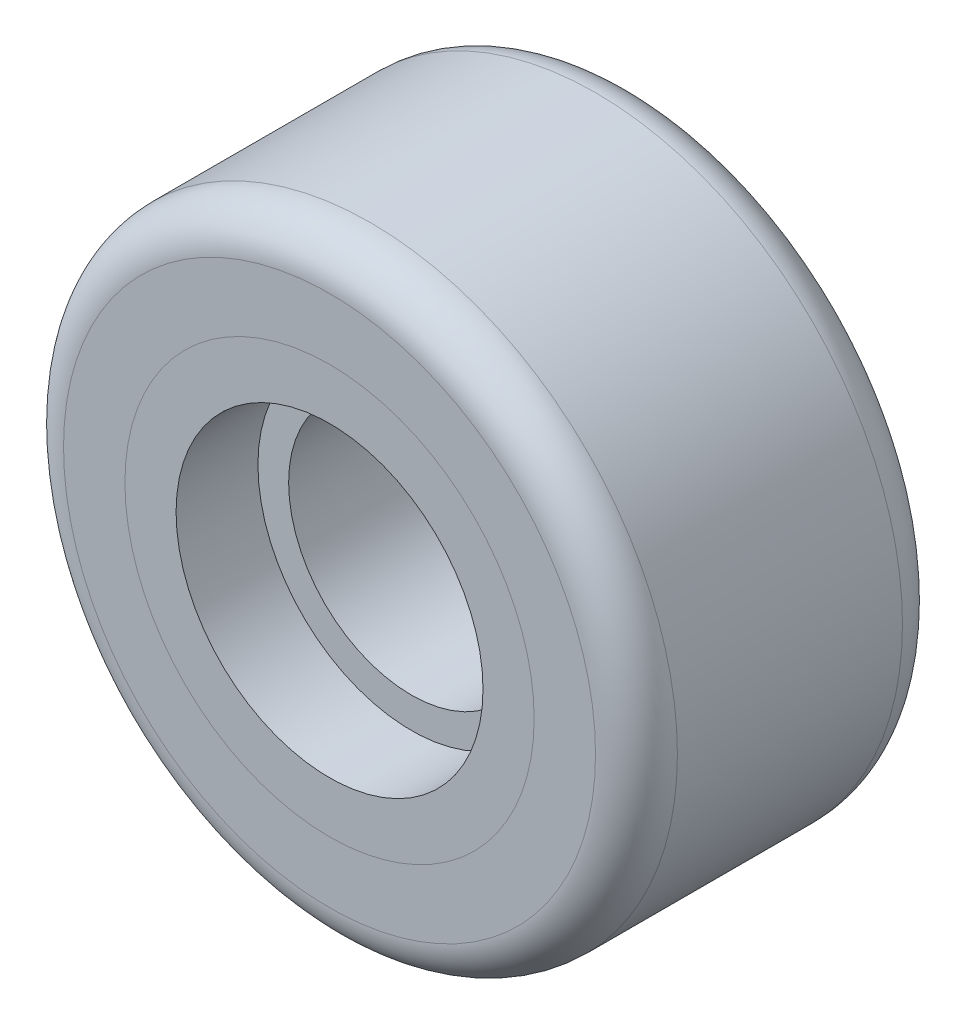
from build123d import *

# Parameters (mm, degrees)
SKETCH1_R           = 10
BOSS_EXTRUDE1_DEPTH = 15
SKETCH2_R           = 15
SKETCH2_R_2         = 10
BOSS_EXTRUDE2_DEPTH = 15
SKETCH3_R           = 6
CUT_EXTRUDE1_DEPTH  = 26.980762114
SKETCH4_R           = 7.5
CUT_EXTRUDE2_DEPTH  = 4
CUT_EXTRUDE3_START  = -4
SKETCH5_R           = 7.5
CUT_EXTRUDE3_DEPTH  = 4
FILLET1_R           = 2


with BuildPart() as part:
    # Sketch1 → Boss-Extrude1 (new body)
    with BuildSketch(Plane.XY):
        Circle(SKETCH1_R)
    extrude(amount=BOSS_EXTRUDE1_DEPTH)

    # Sketch3 → Cut-Extrude1 (cut, through all)
    with BuildSketch(Plane.XY.offset(15)):
        Circle(SKETCH3_R)
    extrude(amount=-CUT_EXTRUDE1_DEPTH, mode=Mode.SUBTRACT)

    # Sketch4 → Cut-Extrude2 (cut)
    with BuildSketch(Plane.XY.offset(15)):
        Circle(SKETCH4_R)
    extrude(amount=-CUT_EXTRUDE2_DEPTH, mode=Mode.SUBTRACT)

    # Sketch5 → Cut-Extrude3 (cut)
    with BuildSketch(Plane(origin=(0, 0, 0), x_dir=(-1, 0, 0), z_dir=(0, 0, -1)).offset(CUT_EXTRUDE3_START)):
        with Locations(Location((0, 0, 0), (0, 0, 180))):
            Circle(SKETCH5_R)
    extrude(amount=CUT_EXTRUDE3_DEPTH, mode=Mode.SUBTRACT)


with BuildPart() as body_2:
    # Sketch2 → Boss-Extrude2 (new body)
    with BuildSketch(Plane.XY.offset(15)):
        Circle(SKETCH2_R)
        Circle(SKETCH2_R_2, mode=Mode.SUBTRACT)
    extrude(amount=-BOSS_EXTRUDE2_DEPTH)

    # Fillet1
    fillet1_edges = [body_2.edges().sort_by_distance(p)[0] for p in [
        (-15, 0, 15),
        (-15, 0, 0),
    ]]
    fillet(fillet1_edges, radius=FILLET1_R)


solid = Compound([part.part, body_2.part])
